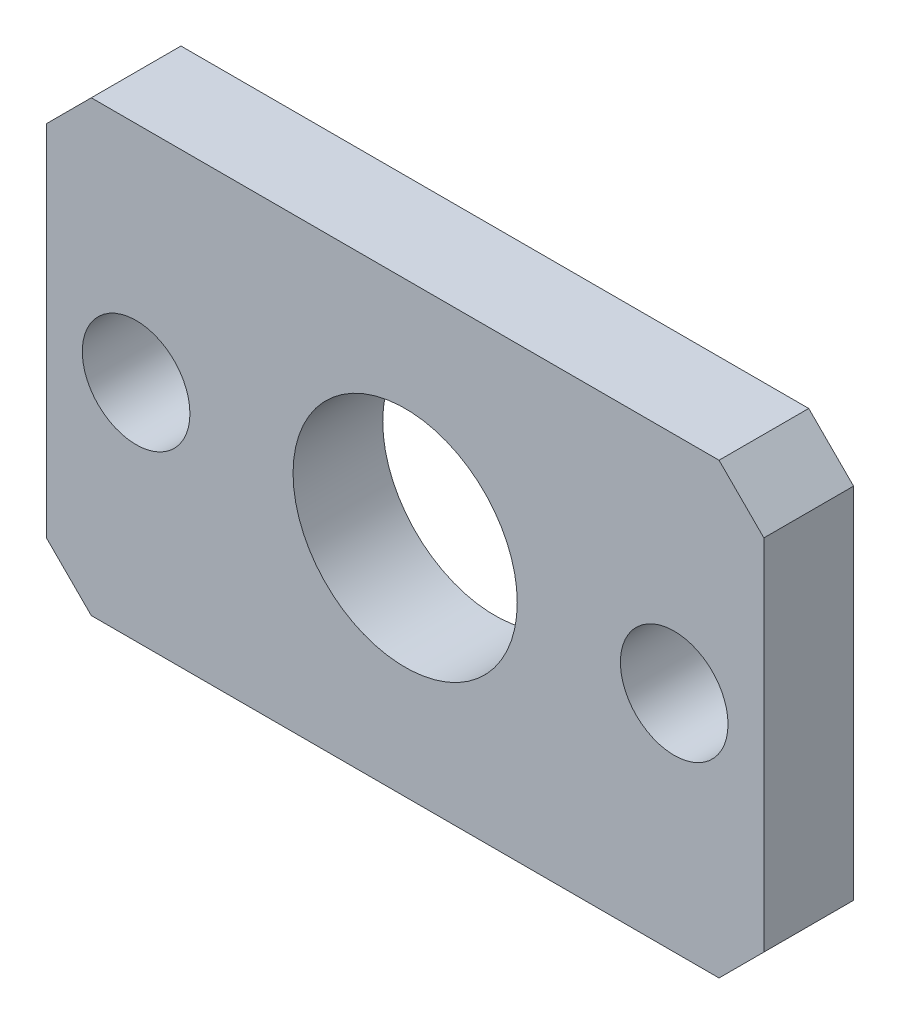
from build123d import *

# Parameters (mm, degrees)
SKETCH1_W           = 8
SKETCH1_H           = 5
BOSS_EXTRUDE1_DEPTH = 0.5
SKETCH2_R           = 1.25
SKETCH2_R_2         = 0.6
CUT_EXTRUDE1_DEPTH  = 5.82182538
CHAMFER1_SIZE       = 0.5


with BuildPart() as part:
    # Sketch1 → Boss-Extrude1 (new, symmetric)
    with BuildSketch(Plane.XY):
        Rectangle(SKETCH1_W, SKETCH1_H)
    extrude(amount=BOSS_EXTRUDE1_DEPTH, both=True)

    # Sketch2 → Cut-Extrude1 (cut, through all)
    with BuildSketch(Plane.XY.offset(0.5)):
        Circle(SKETCH2_R)
        with Locations((-3, 0)):
            Circle(SKETCH2_R_2)
        with Locations((3, 0)):
            Circle(SKETCH2_R_2)
    extrude(amount=-CUT_EXTRUDE1_DEPTH, mode=Mode.SUBTRACT)

    # Chamfer1
    chamfer1_edges = [part.edges().sort_by_distance(p)[0] for p in [
        (4, -2.5, 0),
        (-4, -2.5, 0),
        (-4, 2.5, 0),
        (4, 2.5, 0),
    ]]
    chamfer(chamfer1_edges, length=CHAMFER1_SIZE)


solid = part.part
